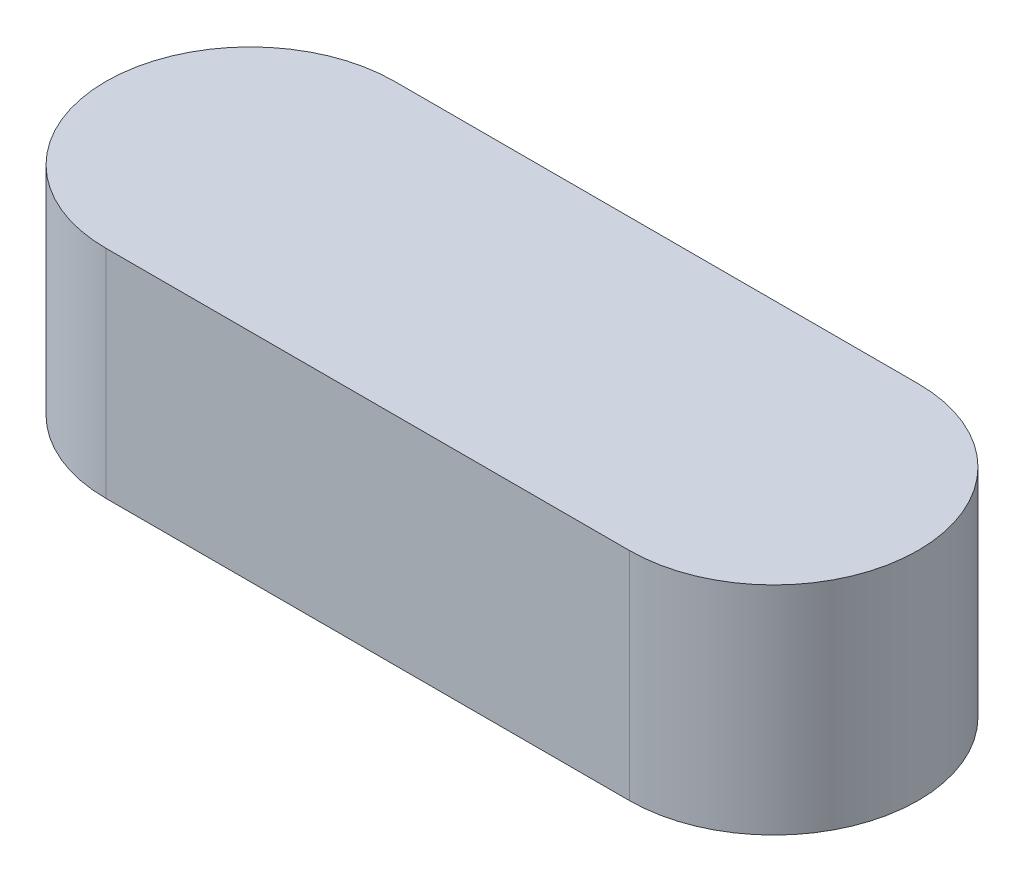
from build123d import *

# Parameters (mm, degrees)
BOSS_EXTRUDE1_DEPTH = 12


with BuildPart() as part:
    # Sketch1 → Boss-Extrude1 (new body)
    with BuildSketch(Plane(origin=(0, 0, 0), x_dir=(1, 0, 0), z_dir=(0, 1, 0))):
        with BuildLine():
            Line((0, 8), (29, 8))
            ThreePointArc((29, 8), (37, 0), (29, -8))
            Line((29, -8), (0, -8))
            ThreePointArc((0, -8), (-8, 0), (0, 8))
        make_face()
    extrude(amount=BOSS_EXTRUDE1_DEPTH)


solid = part.part
